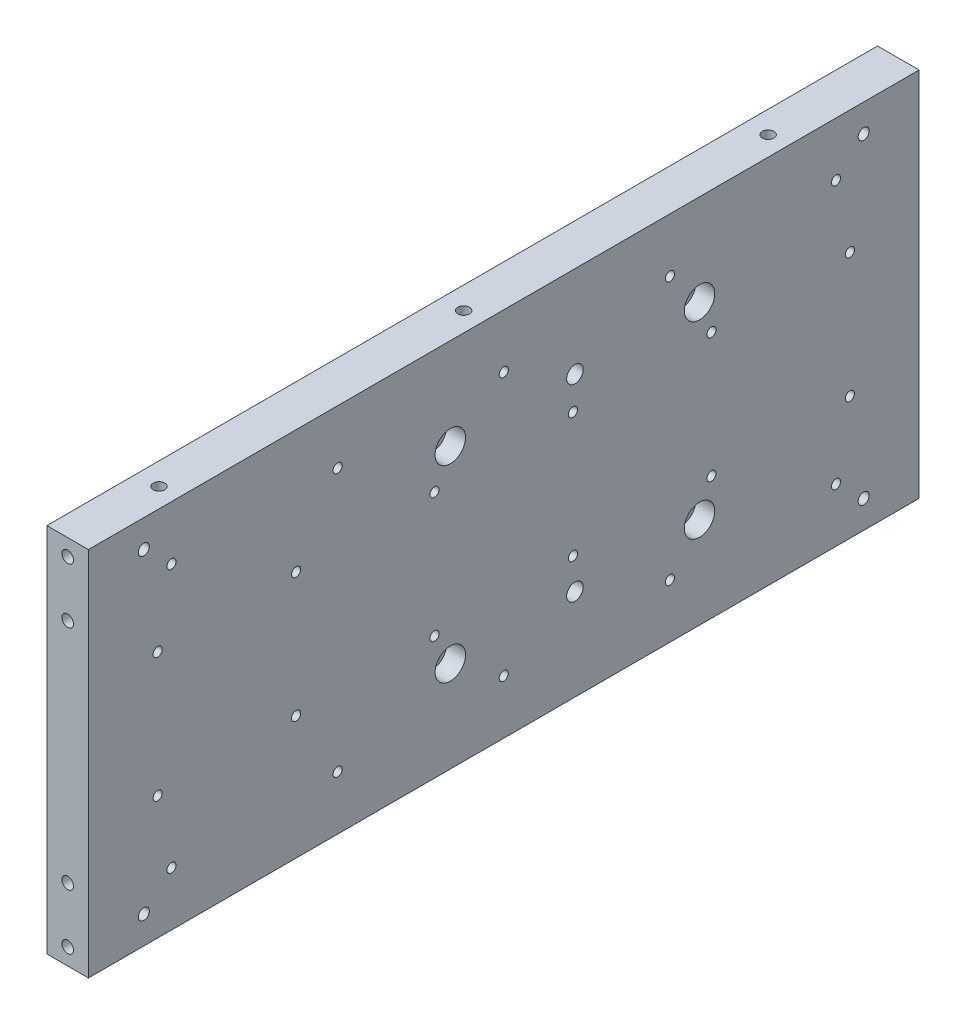
SolidWorks part; units mm, degrees
material "AL6061"
ref_plane "Front Plane" through (0, 0, 0) normal (0, 0, 1) x (1, 0, 0)
ref_plane "Top Plane" through (0, 0, 0) normal (0, 1, 0) x (1, 0, 0)
ref_plane "Right Plane" through (0, 0, 0) normal (1, 0, 0) x (0, 0, -1)
sketch "Sketch1" plane through (0, 0, 0) normal (1, 0, 0) x (0, 0, -1)
  line L1 (-150, -67) -> (150, -67)
  line L2 (-150, -67) -> (-150, 67)
  line L3 (-150, 67) -> (150, 67)
  line L4 (150, -67) -> (150, 67)
  line L5 (-150, -67) -> (150, 67) construction
  line L6 (-150, 67) -> (150, -67) construction
  point P0 (0, 0)
  dimension "D1" = 134
  dimension "D2" = 300
extrude "Boss-Extrude1" add sketch "Sketch1" along normal blind 15
hole_wizard "M4 Tapped Hole1" positions "Sketch2" profile "Sketch3" tap size "M4" standard "GB"
sketch "Sketch2" plane through (15, 0, 0) normal (1, 0, 0) x (0, 0, -1)
  point P0 (-120, -47.5)
  point P3 (-60, -47.5)
  point P6 (0, -47.5)
  point P9 (60, -47.5)
  point P12 (120, -47.5)
  point P25 (120, 47.5)
  point P28 (60, 47.5)
  point P31 (0, 47.5)
  point P34 (-60, 47.5)
  point P37 (-120, 47.5)
sketch "Sketch3" plane through (15, -47.5, 120) normal (0, 1, 0) x (0, 0, -1)
  line L0 (0, 0) -> (0, 11.0914)
  line L1 (0, 11.0914) -> (1.65, 10.1)
  line L2 (1.65, 10.1) -> (1.65, 0)
  line L5 (1.65, 0) -> (0, 0)
  line L10 (0, 11.0914) -> (-1.65, 10.1) construction
  line L11 (0, -6.35) -> (0, 107.95) construction
  dimension "螺纹孔钻头直径" = 3.3
  dimension "螺纹孔钻头深度" = 10.1
  dimension "导头角度" = 118
cosmetic thread "Cosmetic Thread1" parameters "D1"=8, "D2"=4
cosmetic thread "Cosmetic Thread2" parameters "D1"=8, "D2"=4
cosmetic thread "Cosmetic Thread3" parameters "D1"=8, "D2"=4
cosmetic thread "Cosmetic Thread4" parameters "D1"=8, "D2"=4
cosmetic thread "Cosmetic Thread5" parameters "D1"=8, "D2"=4
cosmetic thread "Cosmetic Thread6" parameters "D1"=8, "D2"=4
cosmetic thread "Cosmetic Thread7" parameters "D1"=8, "D2"=4
cosmetic thread "Cosmetic Thread8" parameters "D1"=8, "D2"=4
cosmetic thread "Cosmetic Thread9" parameters "D1"=8, "D2"=4
cosmetic thread "Cosmetic Thread10" parameters "D1"=8, "D2"=4
hole_wizard "M4 Tapped Hole2" positions "Sketch4" profile "Sketch5" tap size "M4" standard "GB"
sketch "Sketch4" plane through (15, 0, 0) normal (1, 0, 0) x (0, 0, -1)
  point P0 (-125, 22.5)
  point P3 (-75, 22.5)
  point P6 (-25, 22.5)
  point P9 (-125, -22.5)
  point P12 (-75, -22.5)
  point P15 (-25, -22.5)
  point P18 (25, 22.5)
  point P21 (75, 22.5)
  point P24 (125, 22.5)
  point P27 (125, -22.5)
  point P30 (75, -22.5)
  point P33 (25, -22.5)
sketch "Sketch5" plane through (15, 22.5, 125) normal (0, 1, 0) x (0, 0, -1)
  line L0 (0, 0) -> (0, 11.0914)
  line L1 (0, 11.0914) -> (1.65, 10.1)
  line L2 (1.65, 10.1) -> (1.65, 0)
  line L5 (1.65, 0) -> (0, 0)
  line L10 (0, 11.0914) -> (-1.65, 10.1) construction
  line L11 (0, -6.35) -> (0, 107.95) construction
  dimension "螺纹孔钻头直径" = 3.3
  dimension "螺纹孔钻头深度" = 10.1
  dimension "导头角度" = 118
cosmetic thread "Cosmetic Thread11" parameters "D1"=8, "D2"=4
cosmetic thread "Cosmetic Thread12" parameters "D1"=8, "D2"=4
cosmetic thread "Cosmetic Thread13" parameters "D1"=8, "D2"=4
cosmetic thread "Cosmetic Thread14" parameters "D1"=8, "D2"=4
cosmetic thread "Cosmetic Thread15" parameters "D1"=8, "D2"=4
cosmetic thread "Cosmetic Thread16" parameters "D1"=8, "D2"=4
cosmetic thread "Cosmetic Thread17" parameters "D1"=8, "D2"=4
cosmetic thread "Cosmetic Thread18" parameters "D1"=8, "D2"=4
cosmetic thread "Cosmetic Thread19" parameters "D1"=8, "D2"=4
cosmetic thread "Cosmetic Thread20" parameters "D1"=8, "D2"=4
cosmetic thread "Cosmetic Thread21" parameters "D1"=8, "D2"=4
cosmetic thread "Cosmetic Thread22" parameters "D1"=8, "D2"=4
hole_wizard "M5 Tapped Hole1" positions "Sketch8" profile "Sketch7" tap size "M5" standard "GB"
sketch "Sketch8" plane through (0, 0, -150) normal (0, 0, -1) x (-1, 0, 0)
  line L3 (-7.5, 67) -> (-7.5, -67) construction
  line L4 (-15, 67) -> (0, 67) construction
  line L5 (-15, -67) -> (0, -67) construction
  line L6 (0, 0) -> (-15, 0) construction
  line L7 (-15, -67) -> (-15, 67) construction
  point P0 (-7.5, -61)
  point P3 (-7.5, -41)
  point P38 (-7.5, 41)
  point P39 (-7.5, 61)
  dimension "D1" = 20
  dimension "D2" = 6
sketch "Sketch7" plane through (7.5, -61, -150) normal (1, 0, 0) x (0, 1, 0)
  line L0 (0, 0) -> (0, 13.6618)
  line L1 (0, 13.6618) -> (2.1, 12.4)
  line L2 (2.1, 12.4) -> (2.1, 0)
  line L5 (2.1, 0) -> (0, 0)
  line L10 (0, 13.6618) -> (-2.1, 12.4) construction
  line L11 (0, -6.35) -> (0, 107.95) construction
  dimension "螺纹孔钻头直径" = 4.2
  dimension "螺纹孔钻头深度" = 12.4
  dimension "导头角度" = 118
cosmetic thread "Cosmetic Thread23" parameters "D1"=10, "D2"=5
cosmetic thread "Cosmetic Thread25" parameters "D1"=10, "D2"=5
cosmetic thread "Cosmetic Thread31" parameters "D1"=10, "D2"=5
cosmetic thread "Cosmetic Thread32" parameters "D1"=10, "D2"=5
mirror "Mirror1" about plane through (0, 0, 0) normal (0, 0, 1) of "M5 Tapped Hole1"
hole_wizard "Ø4.0mm Dowel Hole1" positions "Sketch9" profile "Sketch10" hole size "Ø4.0" standard "GB"
sketch "Sketch9" plane through (15, 0, 0) normal (1, 0, 0) x (0, 0, -1)
  line L0 (150, -67) -> (150, 67) construction
  line L1 (150, 67) -> (-150, 67) construction
  line L2 (0, 0) -> (-150, 0) construction
  line L3 (-150, 67) -> (-150, -67) construction
  line L5 (0, 0) -> (0, 67) construction
  point P2 (130, 57)
  point P24 (-130, 57)
  point P25 (-130, -57)
  point P26 (130, -57)
  dimension "D1" = 20
  dimension "D2" = 10
sketch "Sketch10" plane through (15, 57, -130) normal (0, 1, 0) x (0, 0, -1)
  line L0 (0, 0) -> (0, 7.2017)
  line L1 (0, 7.2017) -> (2, 6)
  line L2 (2, 6) -> (2, 0)
  line L5 (2, 0) -> (0, 0)
  line L10 (0, 7.2017) -> (-2, 6) construction
  line L11 (0, -6.35) -> (0, 107.95) construction
  dimension "孔直径" = 4
  dimension "孔深度" = 6
  dimension "导头角度" = 118
hole_wizard "CBORE for M6 Hexagon socket head cap screws1" positions "Sketch11" profile "Sketch12" counterbore size "M6" standard "GB" end condition through all
sketch "Sketch11" plane through (15, 0, 0) normal (1, 0, 0) x (0, 0, -1)
  point P0 (70.7, 34)
  point P3 (-19.3, 34)
  point P6 (-19.3, -34)
  point P9 (70.7, -34)
sketch "Sketch12" plane through (15, 34, -70.7) normal (0, 1, 0) x (0, 0, -1)
  line L0 (0, 0) -> (0, 15)
  line L1 (0, 15) -> (3.3, 15)
  line L3 (3.3, 15) -> (3.3, 6.8)
  line L4 (3.3, 6.8) -> (5.5, 6.8)
  line L5 (5.5, 6.8) -> (5.5, 0)
  line L7 (5.5, 0) -> (0, 0)
  line L11 (0, -6.35) -> (0, 107.95) construction
  dimension "通孔孔直径" = 6.6
  dimension "通孔孔深度" = 15
  dimension "柱形沉头孔直径" = 11
  dimension "柱形沉头孔深度" = 6.8
hole_wizard "Ø6.0mm Dowel Hole1" positions "Sketch13" profile "Sketch14" hole size "Ø6.0" standard "GB" end condition through all
sketch "Sketch13" plane through (15, 0, 0) normal (1, 0, 0) x (0, 0, -1)
  point P0 (25.7, 34)
  point P3 (25.7, -34)
sketch "Sketch14" plane through (15, 34, -25.7) normal (0, 1, 0) x (0, 0, -1)
  line L0 (0, 0) -> (0, 15)
  line L1 (0, 15) -> (3, 15)
  line L2 (3, 15) -> (3, 0)
  line L5 (3, 0) -> (0, 0)
  line L11 (0, -6.35) -> (0, 107.95) construction
  dimension "通孔孔直径" = 6
  dimension "通孔孔深度" = 15
hole_wizard "M5 Tapped Hole2" positions "Sketch17" profile "Sketch18" tap size "M5" standard "GB"
sketch "Sketch17" plane through (0, 67, 0) normal (0, -1, 0) x (-1, 0, 0)
  line L1 (-15, -150) -> (-15, 150) construction
  line L2 (-15, 150) -> (0, 150) construction
  line L3 (-8, 102.5) -> (-8, -117.5) construction
  point P0 (-8, -117.5)
  point P2 (-8, 102.5)
  point P16 (-8, -7.5)
  dimension "D1" = 220
  dimension "D2" = 47.5
  dimension "D3" = 7
sketch "Sketch18" plane through (8, 67, 117.5) normal (1, 0, 0) x (0, 0, 1)
  line L0 (0, 0) -> (0, 13.6618)
  line L1 (0, 13.6618) -> (2.1, 12.4)
  line L2 (2.1, 12.4) -> (2.1, 0)
  line L5 (2.1, 0) -> (0, 0)
  line L10 (0, 13.6618) -> (-2.1, 12.4) construction
  line L11 (0, -6.35) -> (0, 107.95) construction
  dimension "螺纹孔钻头直径" = 4.2
  dimension "螺纹孔钻头深度" = 12.4
  dimension "导头角度" = 118
cosmetic thread "Cosmetic Thread33" parameters "D1"=10, "D2"=5
cosmetic thread "Cosmetic Thread34" parameters "D1"=10, "D2"=5
cosmetic thread "Cosmetic Thread35" parameters "D1"=10, "D2"=5
